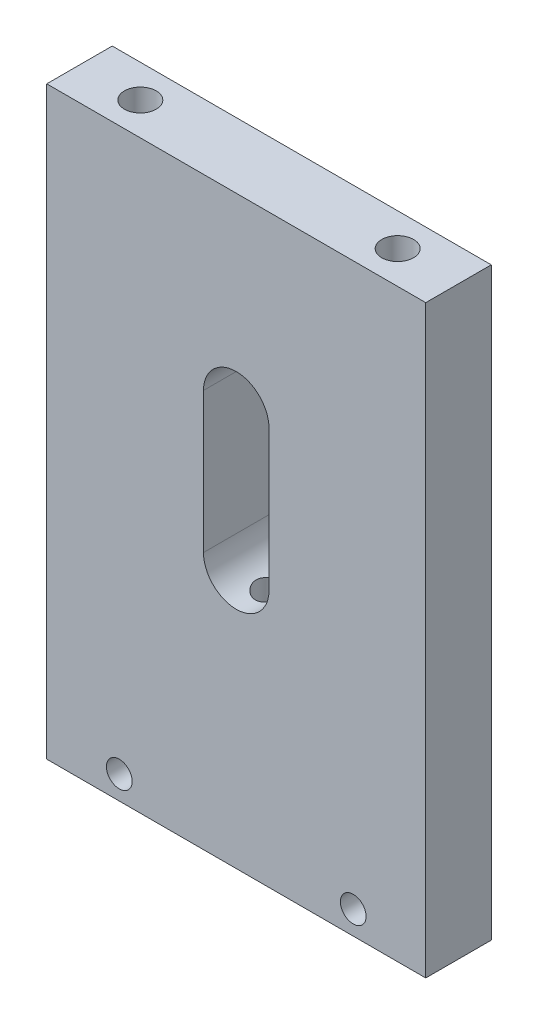
from build123d import *

# Parameters (mm, degrees)
SKETCH_1_W               = 81
SKETCH_1_H               = 125
EXTRUDE_1_DEPTH          = 14
CUT_EXTRUDE_1_DEPTH      = 150.606149606
CUT_EXTRUDE_2_REACH      = 145.948
CUT_EXTRUDE_2_END_RADIUS = 7
SKETCH_4_R               = 3.25
HOLE_WIZARD_M8_1_D       = 6.8
HOLE_WIZARD_M8_1_DEPTH   = 22.25
HOLE_WIZARD_M8_1_TIP     = 2.042926105
SKETCH_11_R              = 2.75
CUT_EXTRUDE_3_DEPTH      = 150.606149699


with BuildPart() as part:
    # 草图1 → 凸台-拉伸1 (new body)
    with BuildSketch(Plane.XY):
        with Locations((40.5, -62.5)):
            Rectangle(SKETCH_1_W, SKETCH_1_H)
    extrude(amount=EXTRUDE_1_DEPTH)

    # 草图2 → 切除-拉伸1 (cut, through all)
    with BuildSketch(Plane.XY.offset(14)):
        with BuildLine():
            Line((33.5, -70), (33.5, -40))
            ThreePointArc((33.5, -40), (40.5, -33), (47.5, -40))
            Line((47.5, -40), (47.5, -70))
            ThreePointArc((47.5, -70), (40.5, -77), (33.5, -70))
        make_face()
    extrude(amount=-CUT_EXTRUDE_1_DEPTH, mode=Mode.SUBTRACT)

    # 切除-拉伸2: up to this cylinder (the profile starts outside it)
    cut_extrude_2_end = Plane(origin=(40.5, -70, 7), z_dir=(0, 0, 1)) * Cylinder(CUT_EXTRUDE_2_END_RADIUS, 306.896, mode=Mode.PRIVATE)
    # 草图4 → 切除-拉伸2 (cut, up to the surface)
    with BuildSketch(Plane(origin=(70, -125, 0), x_dir=(0, 0, -1), z_dir=(0, -1, 0)), mode=Mode.PRIVATE) as cut_extrude_2_sk1:
        with Locations((-7, -29)):
            Circle(SKETCH_4_R)
    cut_extrude_2_tool1 = extrude(cut_extrude_2_sk1.sketch, amount=-CUT_EXTRUDE_2_REACH, mode=Mode.PRIVATE) - cut_extrude_2_end
    add(cut_extrude_2_tool1.solids().sort_by_distance((41, -125, 7))[0], mode=Mode.SUBTRACT)

    # M8 螺纹孔1
    with Locations(Plane(origin=(0, 0, 0), x_dir=(1, 0, 0), z_dir=(0, 1, 0))):
        with Locations((68, -7), (13, -7)):
            Hole(HOLE_WIZARD_M8_1_D / 2, depth=HOLE_WIZARD_M8_1_DEPTH)
            with Locations((0, 0, -(HOLE_WIZARD_M8_1_DEPTH + HOLE_WIZARD_M8_1_TIP / 2))):  # 118° drill point
                Cone(0, HOLE_WIZARD_M8_1_D / 2, HOLE_WIZARD_M8_1_TIP, mode=Mode.SUBTRACT)

    # 草图11 → 切除-拉伸3 (cut, through all)
    with BuildSketch(Plane.XY.offset(14)):
        with Locations((15.5, -120)):
            Circle(SKETCH_11_R)
        with Locations((65.5, -120)):
            Circle(SKETCH_11_R)
    extrude(amount=-CUT_EXTRUDE_3_DEPTH, mode=Mode.SUBTRACT)


solid = part.part
